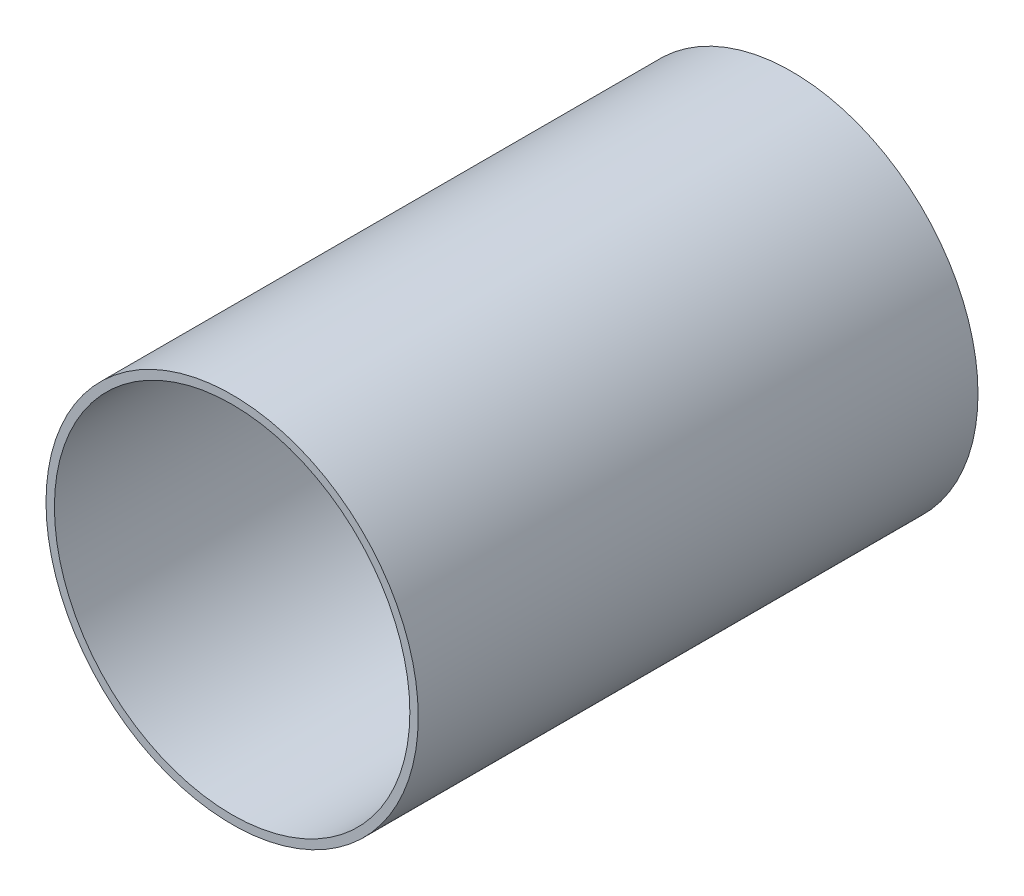
from build123d import *

# Parameters (mm, degrees)
SKETCH1_R           = 66.5
SKETCH1_R_2         = 63.5
BOSS_EXTRUDE1_DEPTH = 200


with BuildPart() as part:
    # Sketch1 → Boss-Extrude1 (new body)
    with BuildSketch(Plane.XY):
        Circle(SKETCH1_R)
        Circle(SKETCH1_R_2, mode=Mode.SUBTRACT)
    extrude(amount=BOSS_EXTRUDE1_DEPTH)


solid = part.part
